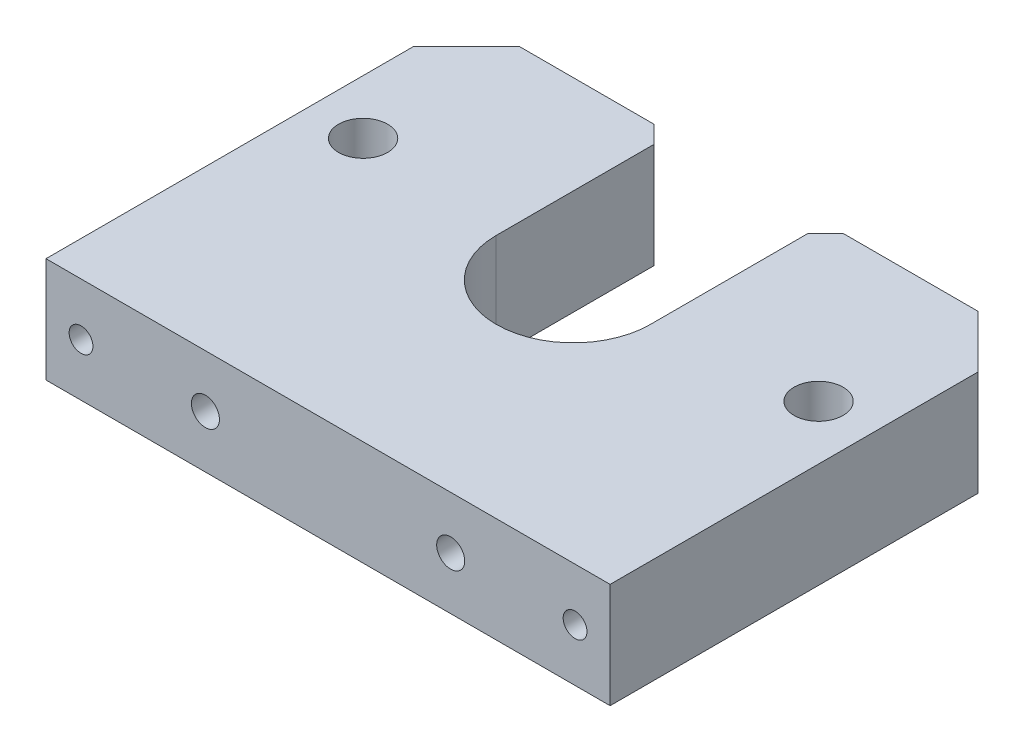
SolidWorks part; units mm, degrees
ref_plane "Front Plane" through (0, 0, 0) normal (0, 0, 1) x (1, 0, 0)
ref_plane "Top Plane" through (0, 0, 0) normal (0, 1, 0) x (1, 0, 0)
ref_plane "Right Plane" through (0, 0, 0) normal (1, 0, 0) x (0, 0, -1)
sketch "Sketch1" plane through (0, 0, 0) normal (0, 1, 0) x (1, 0, 0)
  line L1 (80.5, -60) -> (-80.5, -60)
  line L2 (80.5, -60) -> (80.5, 60)
  line L3 (80.5, 60) -> (-80.5, 60)
  line L4 (-80.5, -60) -> (-80.5, 60)
  line L5 (80.5, -60) -> (-80.5, 60) construction
  line L6 (80.5, 60) -> (-80.5, -60) construction
  point P0 (0, 0)
  dimension "D1" = 120
  dimension "D2" = 161
extrude "Boss-Extrude1" add sketch "Sketch1" along normal blind 30
sketch "Sketch2" plane through (0, 30, 0) normal (0, 1, 0) x (1, 0, 0)
  line L0 (-22, 10) -> (-22, 60)
  line L1 (80.5, 60) -> (-80.5, 60) construction
  line L2 (-22, 60) -> (22, 60)
  line L3 (22, 60) -> (22, 10)
  arc A0 (-22, 10) -> (22, 10) centre (0, 10) ccw
  dimension "D1" = 50
  dimension "D2" = 44
extrude "Cut-Extrude1" cut sketch "Sketch2" against normal through all
hole_wizard "M16 Tapped Hole1" positions "Sketch4" profile "Sketch3" tap size "M16" standard "Iso" end condition through all
sketch "Sketch4" plane through (0, 30, 0) normal (0, 1, 0) x (-1, 0, 0)
  line L0 (22, -60) -> (80.5, -60) construction
  line L1 (-80.5, -60) -> (-22, -60) construction
  point P0 (65, -15)
  point P1 (-65, -15)
  dimension "D1" = 45
  dimension "D2" = 45
  dimension "D3" = 65
  dimension "D4" = 65
cosmetic thread "Cosmetic Thread1" parameters "D2"=16
cosmetic thread "Cosmetic Thread2" parameters "D2"=16
sketch "Sketch3" plane through (-65, 30, -15) normal (1, 0, 0) x (0, 0, 1)
  line L0 (0, 0) -> (0, 30)
  line L1 (0, 30) -> (7, 30)
  line L2 (7, 30) -> (7, 0)
  line L5 (7, 0) -> (0, 0)
  line L11 (0, -6.35) -> (0, 107.95) construction
  dimension "通孔螺纹孔钻头直径" = 14
  dimension "通孔螺纹孔钻头深度" = 30
hole_wizard "M8 Tapped Hole1" positions "Sketch6" profile "Sketch5" tap size "M8" standard "ISO"
sketch "Sketch6" plane through (0, 0, 60) normal (0, 0, 1) x (1, 0, 0)
  line L0 (-80.5, 30) -> (-80.5, 0) construction
  line L1 (80.5, 30) -> (80.5, 0) construction
  line L2 (-80.5, 0) -> (80.5, 0) construction
  point P0 (70.5, 15)
  point P1 (-70.5, 15)
  dimension "D1" = 10
  dimension "D2" = 10
  dimension "D3" = 15
  dimension "D4" = 15
sketch "Sketch5" plane through (70.5, 15, 60) normal (1, 0, 0) x (0, -1, 0)
  line L0 (0, 0) -> (0, 21.7929)
  line L1 (0, 21.7929) -> (3.4, 19.75)
  line L2 (3.4, 19.75) -> (3.4, 0)
  line L5 (3.4, 0) -> (0, 0)
  line L10 (0, 21.7929) -> (-3.4, 19.75) construction
  line L11 (0, -6.35) -> (0, 107.95) construction
  dimension "螺纹孔钻头直径" = 6.8
  dimension "螺纹孔钻头深度" = 19.75
  dimension "导头角度" = 118
cosmetic thread "Cosmetic Thread3" parameters "D1"=16, "D2"=8
cosmetic thread "Cosmetic Thread4" parameters "D1"=16, "D2"=8
sketch "Sketch7" plane through (0, 0, 60) normal (0, 0, 1) x (1, 0, 0)
  line L0 (-80.5, 0) -> (80.5, 0) construction
  circle A0 centre (-35, 15) radius 4
  circle A1 centre (35, 15) radius 4
  dimension "D5" = 8
  dimension "D6" = 8
  dimension "D1" = 15
  dimension "D2" = 15
  dimension "D3" = 35
  dimension "D4" = 35
extrude "Cut-Extrude2" cut sketch "Sketch7" against normal blind 15
chamfer "Chamfer1" distance 15 angle 45 2 edges at (80.5, 15, -60) (-80.5, 15, -60)
chamfer "Chamfer2" distance 5 angle 45 2 edges at (22, 15, -60) (-22, 15, -60)
